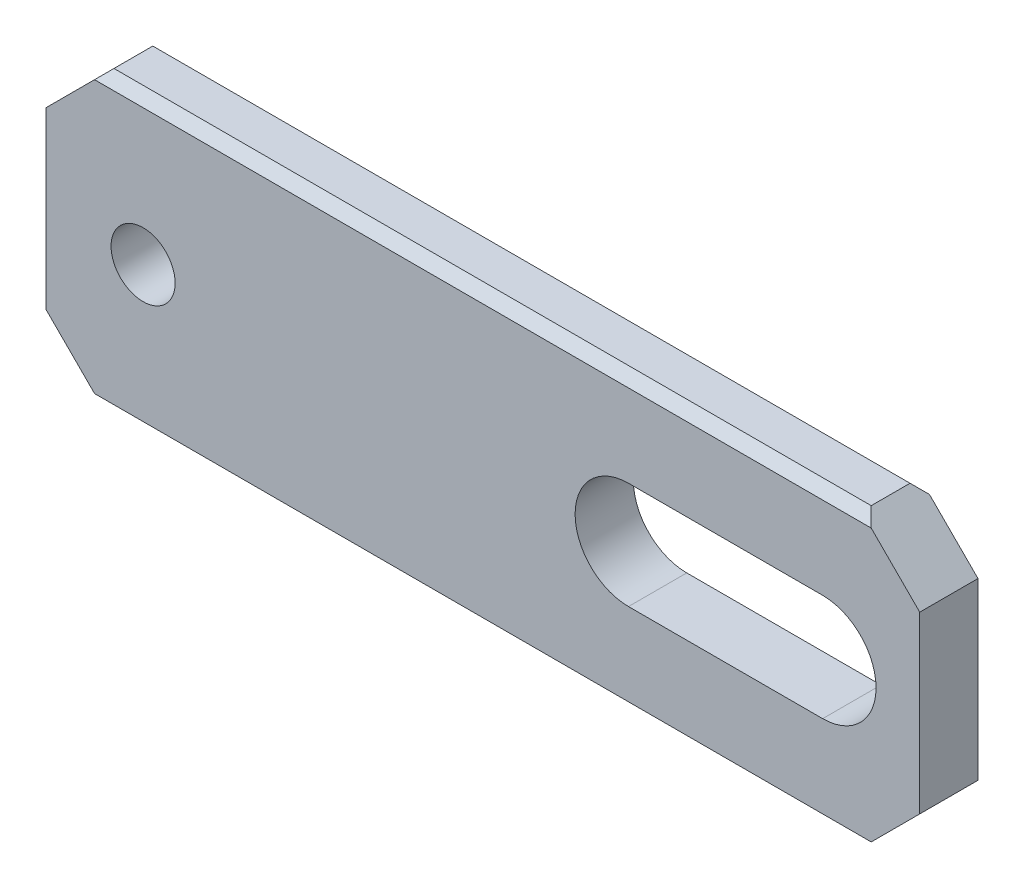
from build123d import *

# Parameters (mm, degrees)
SKETCH1_W             = 45
SKETCH1_H             = 15
BOSS_EXTRUDE1_DEPTH   = 3
M4_TAPPED_HOLE1_D     = 3.3
M4_TAPPED_HOLE1_DEPTH = 10.1
M4_TAPPED_HOLE1_TIP   = 0.991420021
CUT_EXTRUDE1_DEPTH    = 3
CHAMFER1_SIZE         = 3
CHAMFER2_SIZE         = 0.5


with BuildPart() as part:
    # Sketch1 → Boss-Extrude1 (new body)
    with BuildSketch(Plane.XY):
        Rectangle(SKETCH1_W, SKETCH1_H)
    extrude(amount=BOSS_EXTRUDE1_DEPTH)

    # M4 Tapped Hole1
    with Locations(Plane.XY.offset(3)):
        with Locations((-17.5, 0)):
            Hole(M4_TAPPED_HOLE1_D / 2, depth=M4_TAPPED_HOLE1_DEPTH)
            with Locations((0, 0, -(M4_TAPPED_HOLE1_DEPTH + M4_TAPPED_HOLE1_TIP / 2))):  # 118° drill point
                Cone(0, M4_TAPPED_HOLE1_D / 2, M4_TAPPED_HOLE1_TIP, mode=Mode.SUBTRACT)

    # Sketch4 → Cut-Extrude1 (cut)
    with BuildSketch(Plane.XY.offset(3)):
        with BuildLine():
            Line((7.5, 2.75), (17.5, 2.75))
            ThreePointArc((17.5, 2.75), (20.25, 0), (17.5, -2.75))
            Line((17.5, -2.75), (7.5, -2.75))
            ThreePointArc((7.5, -2.75), (4.75, 0), (7.5, 2.75))
        make_face()
    extrude(amount=-CUT_EXTRUDE1_DEPTH, mode=Mode.SUBTRACT)

    # Chamfer1
    chamfer1_edges = [part.edges().sort_by_distance(p)[0] for p in [
        (22.5, -7.5, 1.5),
        (-22.5, -7.5, 1.5),
        (-22.5, 7.5, 1.5),
        (22.5, 7.5, 1.5),
    ]]
    chamfer(chamfer1_edges, length=CHAMFER1_SIZE)

    # Chamfer2
    chamfer2_edges = [part.edges().sort_by_distance(p)[0] for p in [
        (0, -7.5, 0),
        (0, 7.5, 0),
        (0, -7.5, 3),
        (0, 7.5, 3),
    ]]
    chamfer(chamfer2_edges, length=CHAMFER2_SIZE)


solid = part.part
